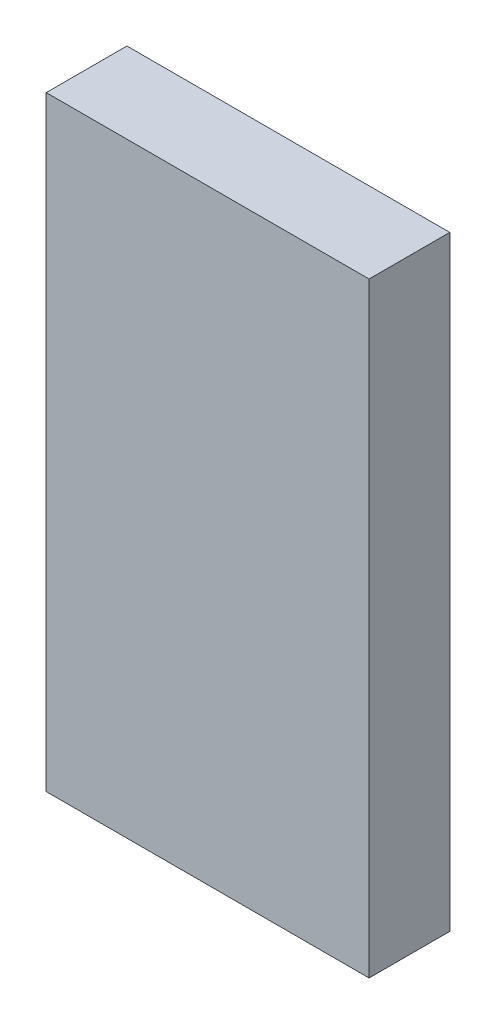
from build123d import *

# Parameters (mm, degrees)
SKETCH1_W           = 80
SKETCH1_H           = 150
BOSS_EXTRUDE1_DEPTH = 20


with BuildPart() as part:
    # Sketch1 → Boss-Extrude1 (new body)
    with BuildSketch(Plane.XY):
        Rectangle(SKETCH1_W, SKETCH1_H)
    extrude(amount=BOSS_EXTRUDE1_DEPTH)


solid = part.part
